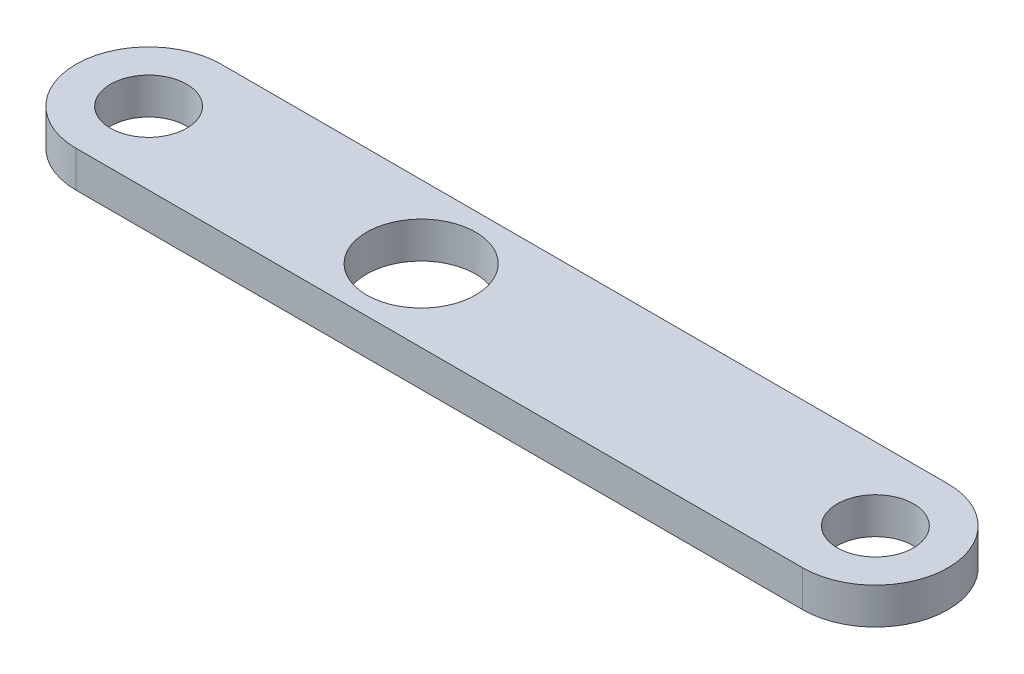
SolidWorks part; units mm, degrees
ref_plane "Front Plane" through (0, 0, 0) normal (0, 0, 1) x (1, 0, 0)
ref_plane "Top Plane" through (0, 0, 0) normal (0, 1, 0) x (1, 0, 0)
ref_plane "Right Plane" through (0, 0, 0) normal (1, 0, 0) x (0, 0, -1)
sketch "Sketch1" plane through (0, 0, 0) normal (0, 1, 0) x (1, 0, 0)
  line L0 (-25.4, 0) -> (25.4, 0) construction
  line L1 (-25.4, 5.08) -> (25.4, 5.08)
  line L2 (-25.4, -5.08) -> (25.4, -5.08)
  arc A0 (-25.4, 5.08) -> (-25.4, -5.08) centre (-25.4, 0) ccw
  arc A1 (25.4, -5.08) -> (25.4, 5.08) centre (25.4, 0) ccw
  circle A2 centre (-25.4, 0) radius 2.667
  circle A3 centre (25.4, 0) radius 2.667
  circle A4 centre (-6.35, 0) radius 3.81
  point P2 (0, 0)
  dimension "D1" = 5.08
  dimension "D3" = 5.334
  dimension "D4" = 5.334
  dimension "D6" = 7.62
  dimension "D2" = 50.8
  dimension "D5" = 19.05
extrude "Boss-Extrude1" add sketch "Sketch1" along normal blind 2.54
scale "Scale1" bodies to scale 101 scale about origin uniform scaling yes scale factor 2
